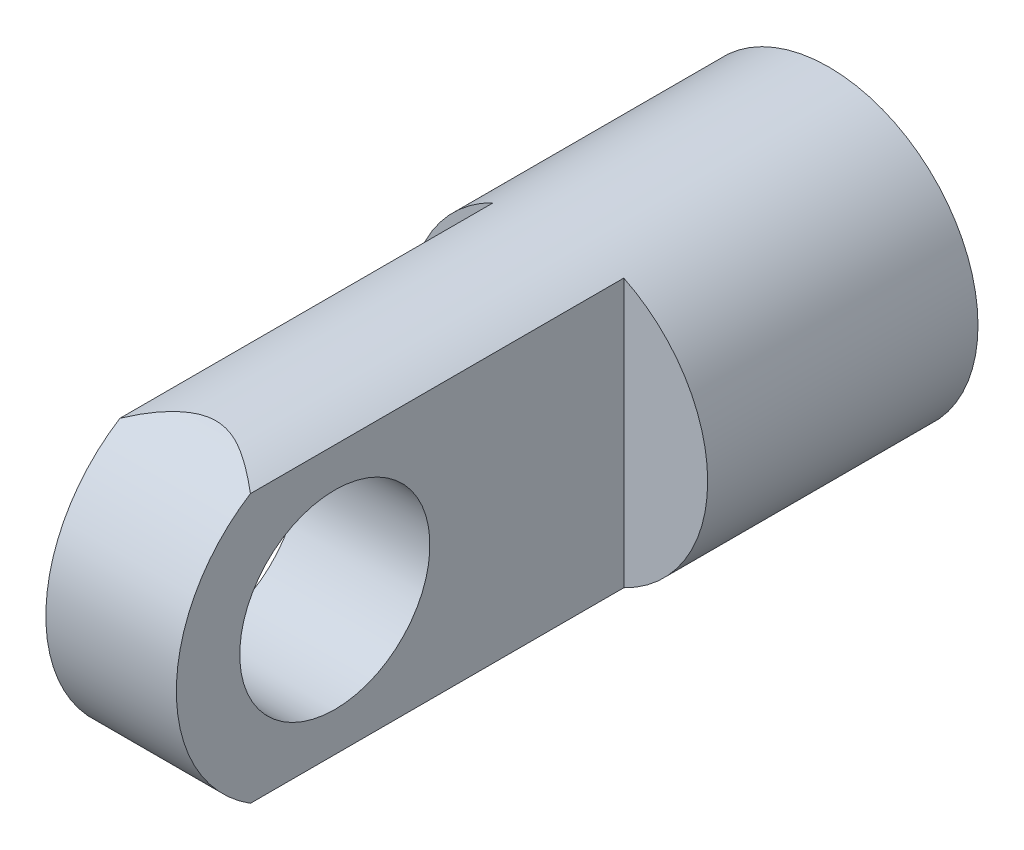
SolidWorks part; units mm, degrees
ref_plane "前视基准面" through (0, 0, 0) normal (0, 0, 1) x (1, 0, 0)
ref_plane "上视基准面" through (0, 0, 0) normal (0, 1, 0) x (1, 0, 0)
ref_plane "右视基准面" through (0, 0, 0) normal (1, 0, 0) x (0, 0, -1)
sketch "草图1" plane through (0, 0, 0) normal (0, 0, 1) x (1, 0, 0)
  circle A0 centre (0, 0) radius 8
  dimension "D1" = 16
extrude "凸台-拉伸1" add sketch "草图1" along normal blind 38.5
sketch "草图2" plane through (0, 0, 38.5) normal (0, 0, 1) x (1, 0, 0)
  line L0 (0, 0) -> (0, 3.9677) construction
  line L1 (0, 0) -> (-10.0086, 0) construction
  line L2 (3.5, 8) -> (3.5, -8)
  line L3 (-8.5, 8) -> (-3.5, 8)
  line L4 (-8.5, 8) -> (-8.5, -8)
  line L5 (-8.5, -8) -> (-3.5, -8)
  line L6 (-3.5, 8) -> (-3.5, -8)
  line L7 (8.5, -8) -> (3.5, -8)
  line L8 (8.5, 8) -> (8.5, -8)
  line L9 (8.5, 8) -> (3.5, 8)
  dimension "D1" = 7
  dimension "D2" = 16
  dimension "D3" = 5
extrude "切除-拉伸1" cut sketch "草图2" against normal blind 24
sketch "草图3" plane through (3.5, 0, 0) normal (1, 0, 0) x (0, 0, -1)
  line L0 (0, -8) -> (0, 8) construction
  circle A0 centre (-30, 0) radius 5.1
  dimension "D1" = 10.2
  dimension "D2" = 30
extrude "切除-拉伸2" cut sketch "草图3" against normal blind 24
sketch "草图4" plane through (3.5, 0, 0) normal (1, 0, 0) x (0, 0, -1)
  line L0 (-30, 8.5) -> (-30, 11)
  line L1 (-30, 11) -> (-45, 11)
  line L2 (-45, 11) -> (-45, -11)
  line L3 (-45, -11) -> (-30, -11)
  line L4 (-30, -11) -> (-30, -8.5)
  line L5 (-30, 0) -> (-45.8256, 0) construction
  arc A0 (-30, 8.5) -> (-30, -8.5) centre (-30, 0) ccw
  dimension "D1" = 17
  dimension "D2" = 22
  dimension "D3" = 15
extrude "切除-拉伸3" cut sketch "草图4" against normal through all
hole_wizard "M8 螺纹孔1" positions "草图5" profile "草图6" tap size "M8" standard "GB"
sketch "草图5" plane through (0, 0, 0) normal (0, 0, -1) x (-1, 0, 0)
  point P0 (0, 0)
sketch "草图6" plane through (0, 0, 0) normal (1, 0, 0) x (0, 1, 0)
  line L0 (0, 0) -> (0, 14.0429)
  line L1 (0, 14.0429) -> (3.4, 12)
  line L2 (3.4, 12) -> (3.4, 0)
  line L5 (3.4, 0) -> (0, 0)
  line L10 (0, 14.0429) -> (-3.4, 12) construction
  line L11 (0, -6.35) -> (0, 107.95) construction
  dimension "螺纹孔钻头直径" = 6.8
  dimension "螺纹孔钻头深度" = 12
  dimension "导头角度" = 118
cosmetic thread "孔螺蚊线1" parameters "D1"=10, "D2"=8
